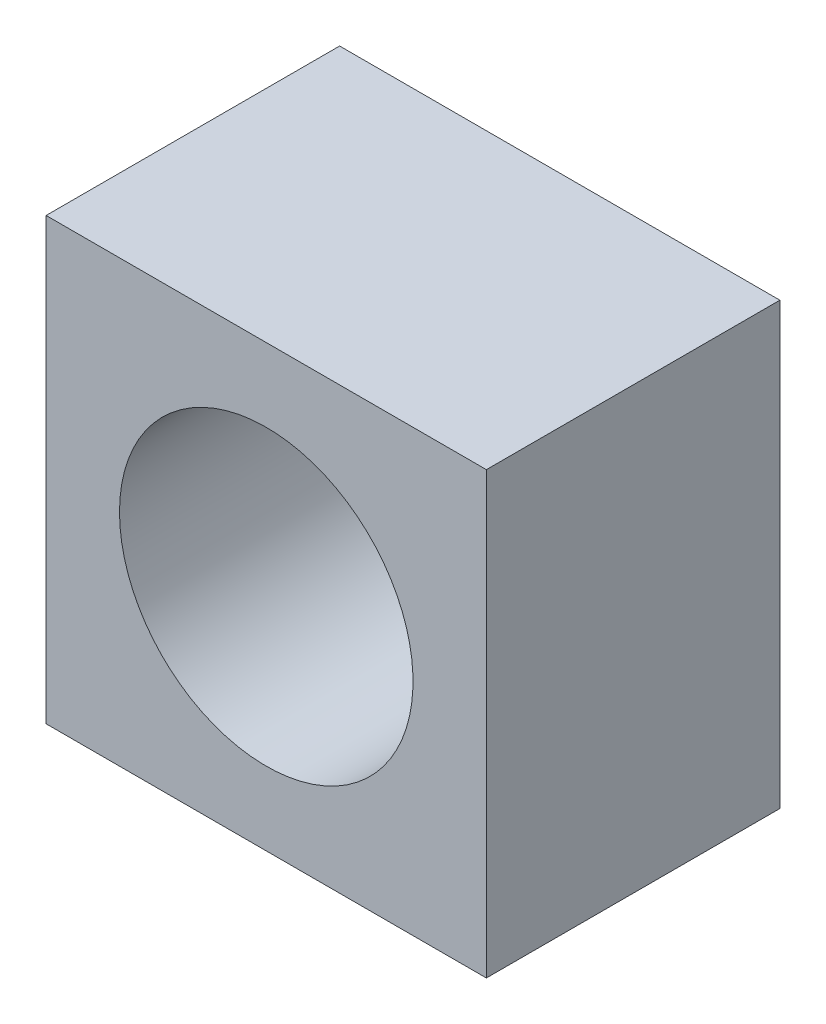
SolidWorks part; units mm, degrees
ref_plane "Front Plane" through (0, 0, 0) normal (0, 0, 1) x (1, 0, 0)
ref_plane "Top Plane" through (0, 0, 0) normal (0, 1, 0) x (1, 0, 0)
ref_plane "Right Plane" through (0, 0, 0) normal (1, 0, 0) x (0, 0, -1)
ref_plane "Plane1" through (0, 0, 10) normal (0, 0, 1) x (1, 0, 0)
sketch "Sketch1" plane through (0, 0, 10) normal (0, 0, 1) x (1, 0, 0)
  line L0 (-15, -15) -> (15, -15)
  line L1 (15, -15) -> (15, 15)
  line L2 (15, 15) -> (-15, 15)
  line L3 (-15, 15) -> (-15, -15)
  circle A0 centre (0, 0) radius 10
extrude "Boss-Extrude1" add sketch "Sketch1" against normal blind 20
